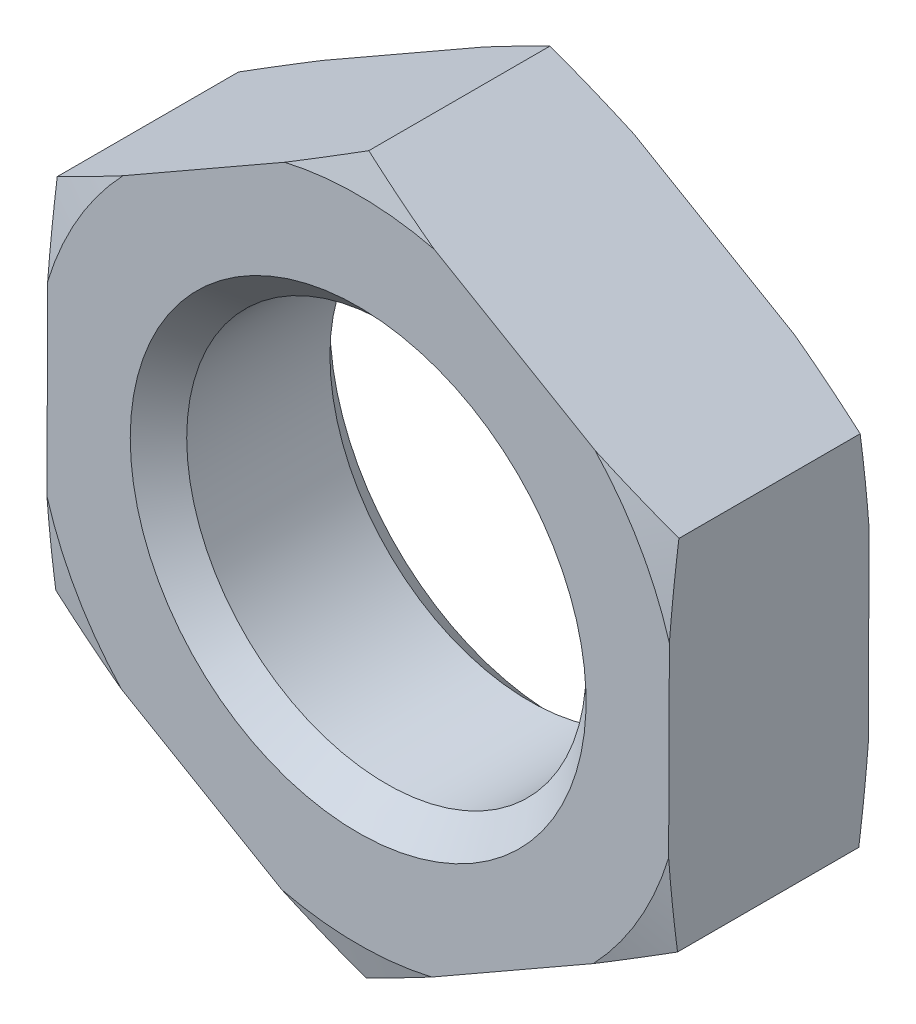
SolidWorks part; units mm, degrees
extrude "基体-拉伸" add sketch "草图1" along normal blind 4
sketch "草图1" plane through (0, 0, 0) normal (0, 0, 1) x (1, 0, 0)
  line L0 (-26.8088, 0) -> (37.1748, 0) construction
  line L1 (0, 25.0215) -> (0, -25.0215) construction
  line L3 (0.0283, 7.1899) -> (-6.2125, 3.6195)
  line L4 (-6.2125, 3.6195) -> (-6.2408, -3.5705)
  line L5 (-6.2408, -3.5705) -> (-0.0283, -7.1899)
  line L6 (-0.0283, -7.1899) -> (6.2125, -3.6195)
  line L7 (6.2125, -3.6195) -> (6.2408, 3.5705)
  line L8 (6.2408, 3.5705) -> (0.0283, 7.1899)
  circle A0 centre (0, 0) radius 6.2267 construction
  circle A1 centre (0, 0) radius 4
cosmetic thread "装饰螺纹线1"
chamfer "倒角1" distance 0.5655 angle 45 2 edges at (4, 0, 0) (4, 0, 4)
material "04级"
ref_plane "基准面1" through (0, 0, 0) normal (0, 0, 1) x (1, 0, 0)
ref_plane "基准面2" through (0, 0, 0) normal (0, 1, 0) x (1, 0, 0)
ref_plane "基准面3" through (0, 0, 0) normal (1, 0, 0) x (0, 0, -1)
sketch "尺寸草图" plane through (0, 0, 0) normal (0, 0, 1) x (1, 0, 0)
  line L0 (0, 0) -> (24.1005, 0)
  line L1 (0, 0) -> (8.75, 0)
  line L2 (46.8781, 0) -> (58.4781, 0)
  line L3 (-7.619, 0) -> (0, 0)
  point P3 (8, 0)
  point P4 (2.5, 0)
  point P5 (14.38, 0)
  point P6 (4, 0)
  point P7 (7.3, 0)
  point P8 (13, 0)
sketch "草图2" plane through (0, 0, 0) normal (0, 0, -1) x (-1, 0, 0)
  circle A0 centre (0, 0) radius 6.5
  circle A1 centre (0, 0) radius 4 construction
extrude "切除-拉伸1" cut sketch "草图2" against normal through all draft 75 flip side to cut
sketch "草图3" plane through (0, 0, 4) normal (0, 0, 1) x (1, 0, 0)
  circle A0 centre (0, 0) radius 6.5
extrude "切除-拉伸2" cut sketch "草图3" against normal through all draft 75 flip side to cut
equation "\"e@草图1\" = \"e@尺寸草图\""
equation "\"D1@尺寸草图\" = \"D@尺寸草图\" / 1.05"
equation "\"D@草图1\" = \"D@尺寸草图\""
equation "\"m@基体-拉伸\" = \"m@尺寸草图\""
equation "\"D1@草图3\" = \"s@尺寸草图\""
equation "\"s@草图2\" = \"s@尺寸草图\""
equation "\"D2@装饰螺纹线1\" = 1.05 * \"D1@尺寸草图\""
equation "\"D1@倒角1\" =  ( \"da@尺寸草图\" - \"D1@尺寸草图\" )  / 2"
